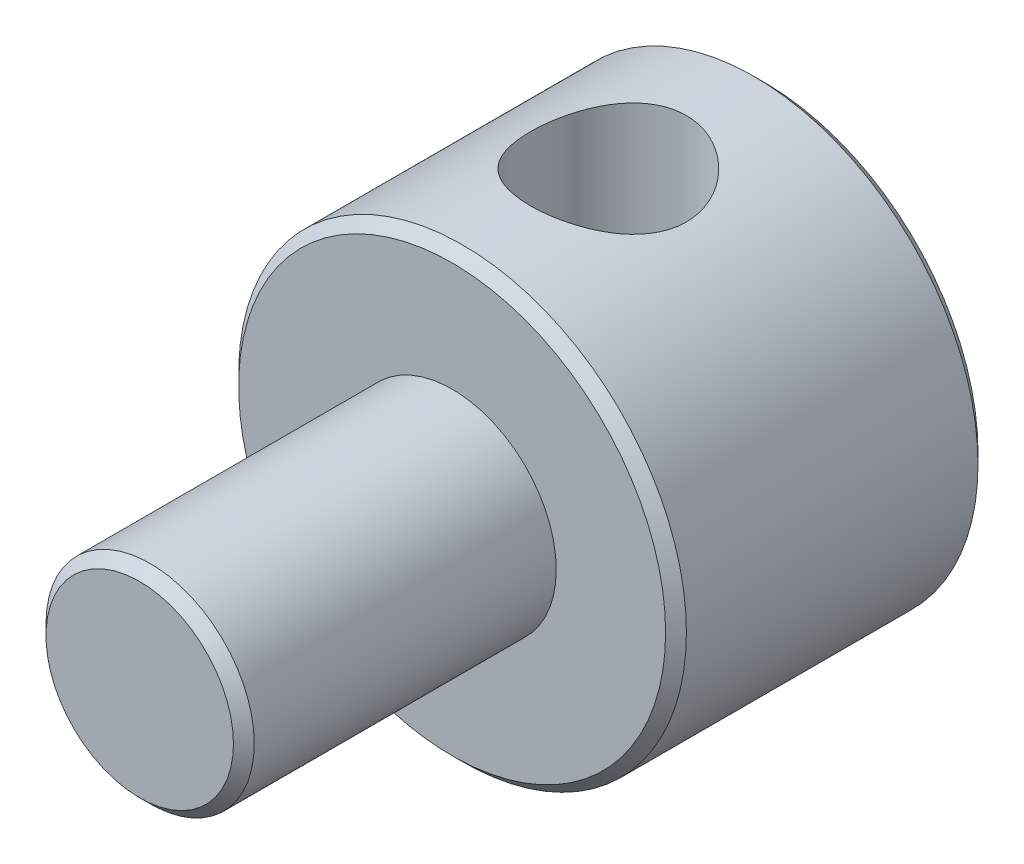
from build123d import *

# Parameters (mm, degrees)
SKETCH1_R                = 4.3
BOSS_EXTRUDE1_DEPTH      = 6
SKETCH2_R                = 2
BOSS_EXTRUDE2_DEPTH      = 6
CHAMFER1_SIZE            = 0.2
F_3_0_3_DIAMETER_HOLE1_D = 3


with BuildPart() as part:
    # Sketch1 → Boss-Extrude1 (new body)
    with BuildSketch(Plane.XY):
        Circle(SKETCH1_R)
    extrude(amount=BOSS_EXTRUDE1_DEPTH)

    # Sketch2 → Boss-Extrude2 (add)
    with BuildSketch(Plane.XY.offset(6)):
        Circle(SKETCH2_R)
    extrude(amount=BOSS_EXTRUDE2_DEPTH)

    # Chamfer1
    chamfer1_edges = [part.edges().sort_by_distance(p)[0] for p in [
        (-4.3, 0, 0),
        (-4.3, 0, 6),
        (-2, 0, 12),
    ]]
    chamfer(chamfer1_edges, length=CHAMFER1_SIZE)

    # Ø3.0 (3) Diameter Hole1 (through all)
    with Locations(Plane(origin=(0, 5, 0), x_dir=(1, 0, 0), z_dir=(0, 1, 0))):
        with Locations((0, -3)):
            Hole(F_3_0_3_DIAMETER_HOLE1_D / 2)


solid = part.part
